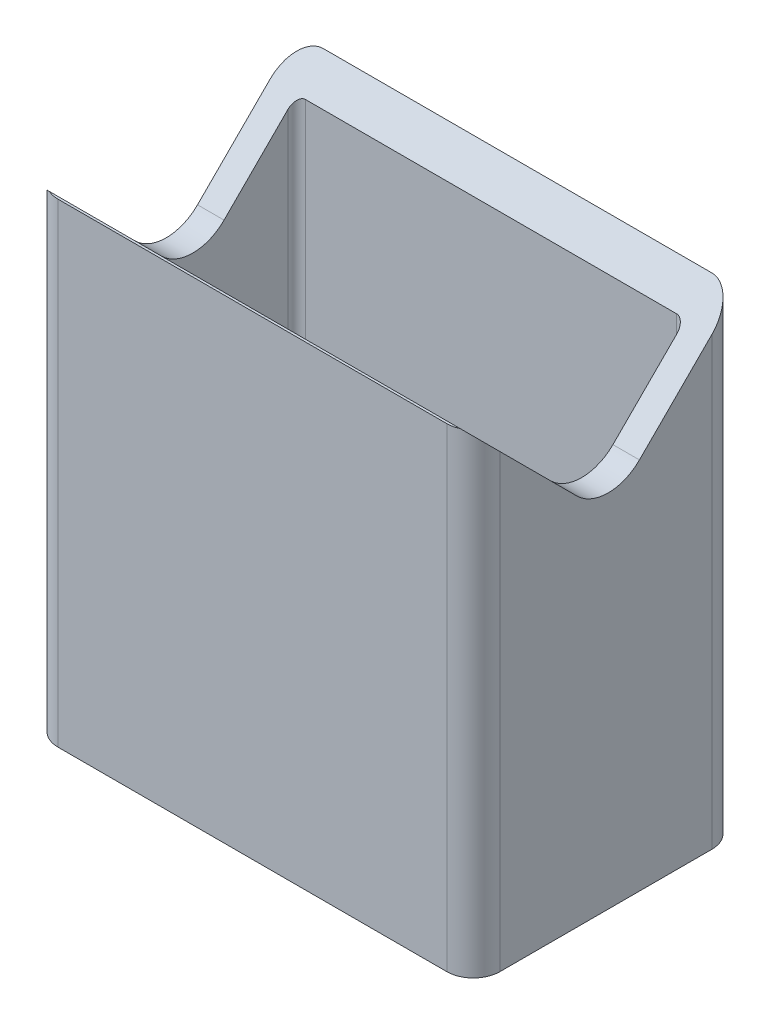
from build123d import *

# Parameters (mm, degrees)
SKETCH1_W           = 50
SKETCH1_H           = 53.7
BOSS_EXTRUDE1_DEPTH = 30
SHELL1_T            = -3
CUT_EXTRUDE1_DEPTH  = 66
FILLET1_R           = 3
FILLET2_R           = 1


with BuildPart() as part:
    # Sketch1 → Boss-Extrude1 (new body)
    with BuildSketch(Plane.XY):
        Rectangle(SKETCH1_W, SKETCH1_H)
    extrude(amount=BOSS_EXTRUDE1_DEPTH)

    # Shell1
    shell1_openings = [part.faces().sort_by_distance(p)[0] for p in [
        (0, -26.85, 15),
        (0, 26.85, 15),
    ]]
    offset(amount=SHELL1_T, openings=shell1_openings, kind=Kind.INTERSECTION)

    # Sketch2 → Cut-Extrude1 (cut)
    with BuildSketch(Plane(origin=(25, 0, 0), x_dir=(0, 0, -1), z_dir=(1, 0, 0))):
        with BuildLine():
            Line((-11.212154068, 15.401262658), (13.536583273, 40.15))
            Line((13.536583273, 40.15), (-14.747687974, 68.434271247))
            Line((-14.747687974, 68.434271247), (-43.031959221, 40.15))
            Line((-43.031959221, 40.15), (-18.28322188, 15.401262658))
            ThreePointArc((-18.28322188, 15.401262658), (-14.747687974, 13.936796564), (-11.212154068, 15.401262658))
        make_face()
    extrude(amount=-CUT_EXTRUDE1_DEPTH, mode=Mode.SUBTRACT)

    # Fillet1
    fillet1_edges = [part.edges().sort_by_distance(p)[0] for p in [
        (-25, -0.118291637, 0),
        (25, -0.118291637, 0),
        (-25, 0, 30),
        (25, 0, 30),
    ]]
    fillet(fillet1_edges, radius=FILLET1_R)

    # Fillet2
    fillet2_edges = [part.edges().sort_by_distance(p)[0] for p in [
        (22, -1.618291637, 3),
        (22, -1.365979611, 27),
        (-22, -1.618291637, 3),
        (-22, -1.365979611, 27),
    ]]
    fillet(fillet2_edges, radius=FILLET2_R)


solid = part.part
